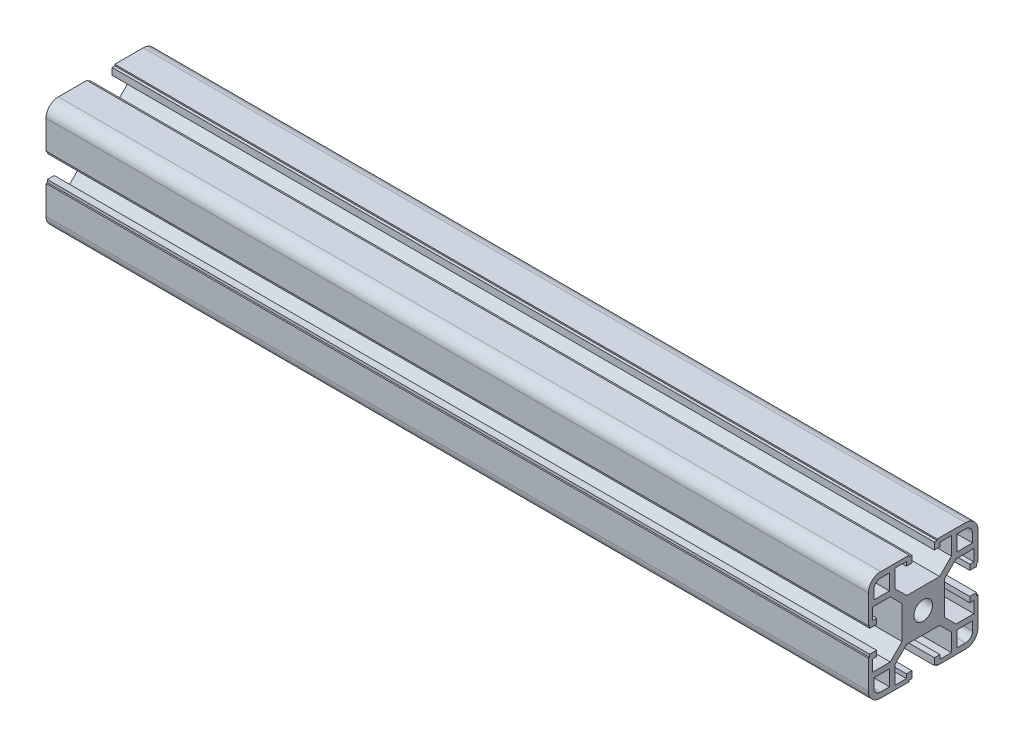
from build123d import *

# Parameters (mm, degrees)
SKETCH1_R                                 = 3.4
ALUMINIUM_PROFILE_40_X_40B_X_R4_5_1_DEPTH = 300


with BuildPart() as part:
    # Sketch1 → Aluminium profile 40 X 40B X R4.5(1) (new body)
    with BuildSketch(Plane.YZ.offset(-984.974958264)):
        with BuildLine():
            Line((-5.1, 20), (-5.1, 19.5))
            Line((-5.1, 19.5), (-4.1, 19.5))
            Line((-4.1, 19.5), (-4.1, 17))
            Line((-4.1, 17), (-6.1, 17))
            Line((-6.1, 17), (-6.1, 18.5))
            Line((-6.1, 18.5), (-10.3, 18.5))
            Line((-10.3, 18.5), (-10.3, 12))
            Line((-10.3, 12), (-6, 7.7))
            Line((-6, 7.7), (6, 7.7))
            Line((6, 7.7), (10.3, 12))
            Line((10.3, 12), (10.3, 18.5))
            Line((10.3, 18.5), (6.1, 18.5))
            Line((6.1, 18.5), (6.1, 17))
            Line((6.1, 17), (4.1, 17))
            Line((4.1, 17), (4.1, 19.5))
            Line((4.1, 19.5), (5.1, 19.5))
            Line((5.1, 19.5), (5.1, 20))
            Line((5.1, 20), (15.5, 20))
            ThreePointArc((15.5, 20), (18.681980515, 18.681980515), (20, 15.5))
            Line((20, 15.5), (20, 5.1))
            Line((20, 5.1), (19.5, 5.1))
            Line((19.5, 5.1), (19.5, 4.1))
            Line((19.5, 4.1), (17, 4.1))
            Line((17, 4.1), (17, 6.1))
            Line((17, 6.1), (18.5, 6.1))
            Line((18.5, 6.1), (18.5, 10.3))
            Line((18.5, 10.3), (12, 10.3))
            Line((12, 10.3), (7.7, 6))
            Line((7.7, 6), (7.7, -6))
            Line((7.7, -6), (12, -10.3))
            Line((12, -10.3), (18.5, -10.3))
            Line((18.5, -10.3), (18.5, -6.1))
            Line((18.5, -6.1), (17, -6.1))
            Line((17, -6.1), (17, -4.1))
            Line((17, -4.1), (19.5, -4.1))
            Line((19.5, -4.1), (19.5, -5.1))
            Line((19.5, -5.1), (20, -5.1))
            Line((20, -5.1), (20, -15.5))
            ThreePointArc((20, -15.5), (18.681980515, -18.681980515), (15.5, -20))
            Line((15.5, -20), (5.1, -20))
            Line((5.1, -20), (5.1, -19.5))
            Line((5.1, -19.5), (4.1, -19.5))
            Line((4.1, -19.5), (4.1, -17))
            Line((4.1, -17), (6.1, -17))
            Line((6.1, -17), (6.1, -18.5))
            Line((6.1, -18.5), (10.3, -18.5))
            Line((10.3, -18.5), (10.3, -12))
            Line((10.3, -12), (6, -7.7))
            Line((6, -7.7), (-6, -7.7))
            Line((-6, -7.7), (-10.3, -12))
            Line((-10.3, -12), (-10.3, -18.5))
            Line((-10.3, -18.5), (-6.1, -18.5))
            Line((-6.1, -18.5), (-6.1, -17))
            Line((-6.1, -17), (-4.1, -17))
            Line((-4.1, -17), (-4.1, -19.5))
            Line((-4.1, -19.5), (-5.1, -19.5))
            Line((-5.1, -19.5), (-5.1, -20))
            Line((-5.1, -20), (-15.5, -20))
            ThreePointArc((-15.5, -20), (-18.681980515, -18.681980515), (-20, -15.5))
            Line((-20, -15.5), (-20, -5.1))
            Line((-20, -5.1), (-19.5, -5.1))
            Line((-19.5, -5.1), (-19.5, -4.1))
            Line((-19.5, -4.1), (-17, -4.1))
            Line((-17, -4.1), (-17, -6.1))
            Line((-17, -6.1), (-18.5, -6.1))
            Line((-18.5, -6.1), (-18.5, -10.3))
            Line((-18.5, -10.3), (-12, -10.3))
            Line((-12, -10.3), (-7.7, -6))
            Line((-7.7, -6), (-7.7, 6))
            Line((-7.7, 6), (-12, 10.3))
            Line((-12, 10.3), (-18.5, 10.3))
            Line((-18.5, 10.3), (-18.5, 6.1))
            Line((-18.5, 6.1), (-17, 6.1))
            Line((-17, 6.1), (-17, 4.1))
            Line((-17, 4.1), (-19.5, 4.1))
            Line((-19.5, 4.1), (-19.5, 5.1))
            Line((-19.5, 5.1), (-20, 5.1))
            Line((-20, 5.1), (-20, 15.5))
            ThreePointArc((-20, 15.5), (-18.681980515, 18.681980515), (-15.5, 20))
            Line((-15.5, 20), (-5.1, 20))
        make_face()
        Circle(SKETCH1_R, mode=Mode.SUBTRACT)
        with BuildLine():
            Line((12.3, 18), (15.5, 18))
            ThreePointArc((15.5, 18), (17.267766953, 17.267766953), (18, 15.5))
            Line((18, 15.5), (18, 12.3))
            Line((18, 12.3), (12.3, 12.3))
            Line((12.3, 12.3), (12.3, 18))
        make_face(mode=Mode.SUBTRACT)
        with BuildLine():
            Line((-15.5, 18), (-12.3, 18))
            Line((-12.3, 18), (-12.3, 12.3))
            Line((-12.3, 12.3), (-18, 12.3))
            Line((-18, 12.3), (-18, 15.5))
            ThreePointArc((-18, 15.5), (-17.267766953, 17.267766953), (-15.5, 18))
        make_face(mode=Mode.SUBTRACT)
        with BuildLine():
            Line((-18, -12.3), (-12.3, -12.3))
            Line((-12.3, -12.3), (-12.3, -18))
            Line((-12.3, -18), (-15.5, -18))
            ThreePointArc((-15.5, -18), (-17.267766953, -17.267766953), (-18, -15.5))
            Line((-18, -15.5), (-18, -12.3))
        make_face(mode=Mode.SUBTRACT)
        with BuildLine():
            Line((12.3, -12.3), (18, -12.3))
            Line((18, -12.3), (18, -15.5))
            ThreePointArc((18, -15.5), (17.267766953, -17.267766953), (15.5, -18))
            Line((15.5, -18), (12.3, -18))
            Line((12.3, -18), (12.3, -12.3))
        make_face(mode=Mode.SUBTRACT)
    extrude(amount=ALUMINIUM_PROFILE_40_X_40B_X_R4_5_1_DEPTH)


solid = part.part
